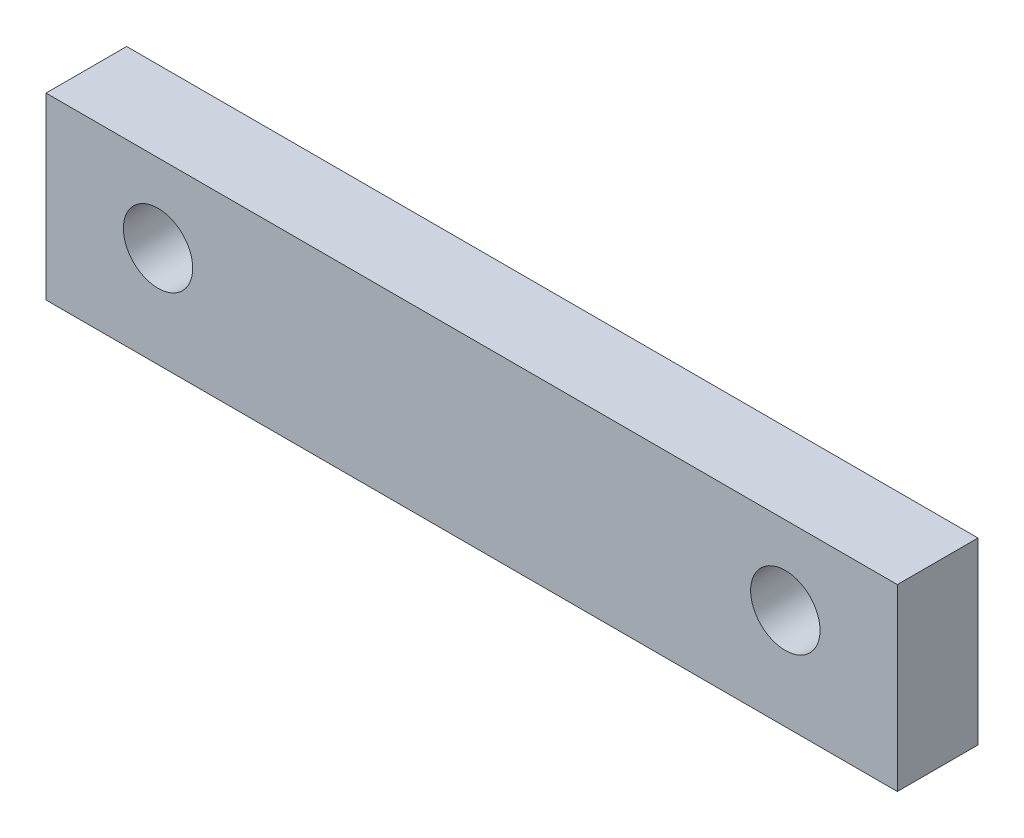
SolidWorks part; units mm, degrees
material "普通碳钢"
ref_plane "Front Plane" through (0, 0, 0) normal (0, 0, 1) x (1, 0, 0)
ref_plane "Top Plane" through (0, 0, 0) normal (0, 1, 0) x (1, 0, 0)
ref_plane "Right Plane" through (0, 0, 0) normal (1, 0, 0) x (0, 0, -1)
sketch "Sketch1" plane through (0, 0, 0) normal (0, 0, 1) x (1, 0, 0)
  line L1 (-190, 40) -> (190, 40)
  line L2 (-190, 40) -> (-190, -40)
  line L3 (-190, -40) -> (190, -40)
  line L4 (190, 40) -> (190, -40)
  dimension "D1" = 80
  dimension "D2" = 380
  dimension "D3" = 40
  dimension "D4" = 190
extrude "Boss-Extrude1" add sketch "Sketch1" along normal mid plane 36
hole_wizard "1-3/8-6 Tapped Hole1" positions "Sketch3" profile "Sketch2" tap size "1-3/8-6" standard "Ansi Inch" end condition through all
sketch "Sketch3" plane through (0, 0, 18) normal (0, 0, 1) x (1, 0, 0)
  line L0 (-190, 40) -> (-190, -40) construction
  line L1 (190, 40) -> (-190, 40) construction
  line L2 (190, -40) -> (190, 40) construction
  point P0 (-140, 5)
  point P1 (140, 5)
  dimension "D1" = 50
  dimension "D2" = 35
  dimension "D3" = 35
  dimension "D4" = 50
sketch "Sketch2" plane through (-140, 5, 18) normal (1, 0, 0) x (0, -1, 0)
  line L0 (0, 0) -> (0, 36)
  line L1 (0, 36) -> (15.4788, 36)
  line L2 (15.4788, 36) -> (15.4788, 0)
  line L5 (15.4788, 0) -> (0, 0)
  line L11 (0, -6.35) -> (0, 107.95) construction
  dimension "通孔螺纹孔钻头直径" = 30.9575
  dimension "通孔螺纹孔钻头深度" = 36
cosmetic thread "Cosmetic thread1"
cosmetic thread "Cosmetic thread2"
